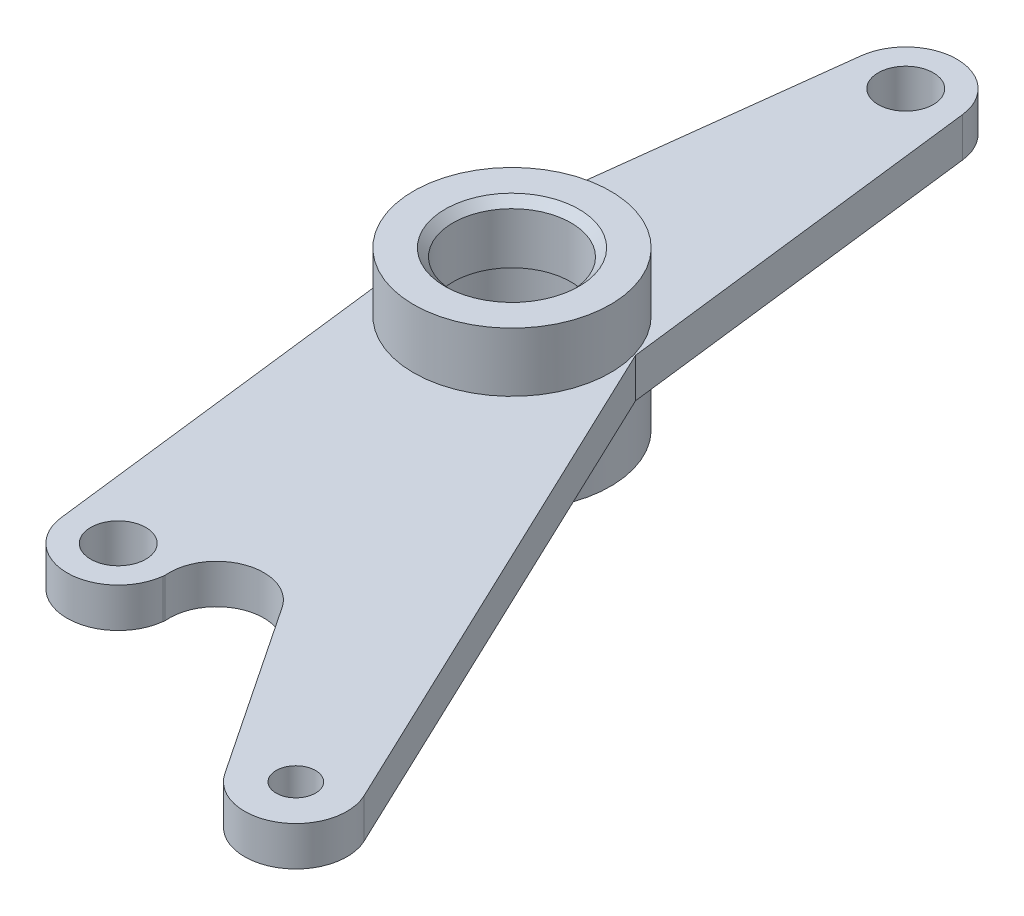
SolidWorks part; units mm, degrees
material "A3"
ref_plane "前视基准面" through (0, 0, 0) normal (0, 0, 1) x (1, 0, 0)
ref_plane "上视基准面" through (0, 0, 0) normal (0, 1, 0) x (1, 0, 0)
ref_plane "右视基准面" through (0, 0, 0) normal (1, 0, 0) x (0, 0, -1)
sketch "草图1" plane through (0, 0, 0) normal (0, 1, 0) x (1, 0, 0)
  circle A0 centre (0, 0) radius 25
  circle A1 centre (0, 0) radius 15
  dimension "D1" = 50
  dimension "D2" = 30
extrude "凸台-拉伸1" add sketch "草图1" along normal mid plane 40
sketch "草图2" plane through (0, 0, 0) normal (0, 1, 0) x (1, 0, 0)
  line L0 (0, 0) -> (0, 100) construction
  line L1 (0, 0) -> (15, 0) construction
  line L2 (-12.9061, 101.56) -> (-24.8193, 3)
  line L3 (12.9061, 101.56) -> (24.3302, 7.0464)
  line L4 (-12.9061, -101.56) -> (-24.8193, -3)
  line L5 (12.9061, -101.56) -> (12.9686, -101.0422)
  line L6 (0, 0) -> (24.918, -99.9405) construction
  line L7 (0, 0) -> (75, -129.9038) construction
  line L8 (24.3302, 7.0464) -> (86.7422, -124.3253)
  line L9 (64.1902, -137.1252) -> (34.8962, -93.2746)
  circle A0 centre (0, 0) radius 25 construction
  arc A1 (-24.8193, 3) -> (-24.8193, -3) centre (0, 0) ccw
  circle A2 centre (0, 0) radius 15 construction
  circle A3 centre (0, 0) radius 15
  circle A4 centre (0, 100) radius 7
  arc A5 (12.9061, 101.56) -> (-12.9061, 101.56) centre (0, 100) ccw
  arc A6 (12.9061, -101.56) -> (-12.9061, -101.56) centre (0, -100) cw
  circle A7 centre (0, -100) radius 7
  arc A8 (34.8962, -93.2746) -> (12.9686, -101.0422) centre (24.918, -99.9405) ccw
  circle A9 centre (75, -129.9038) radius 5
  arc A10 (64.1902, -137.1252) -> (86.7422, -124.3253) centre (75, -129.9038) ccw
  dimension "D2" = 14
  dimension "D3" = 26
  dimension "D8" = 24
  dimension "D9" = 10
  dimension "D10" = 26
  dimension "D1" = 100
  dimension "D4" = 103
  dimension "D5" = 150
  dimension "D6" = 14
  dimension "D7" = 30
extrude "凸台-拉伸2" add sketch "草图2" along normal mid plane 10
chamfer "倒角1" distance 2 angle 45 2 edges at (0, -20, 15) (0, 20, 15)
sketch "草图3" plane through (0, 5, 0) normal (0, 1, 0) x (1, 0, 0)
  circle A0 centre (0, 0) radius 17
  dimension "D1" = 34
extrude "切除-拉伸1" cut sketch "草图3" against normal blind 10
